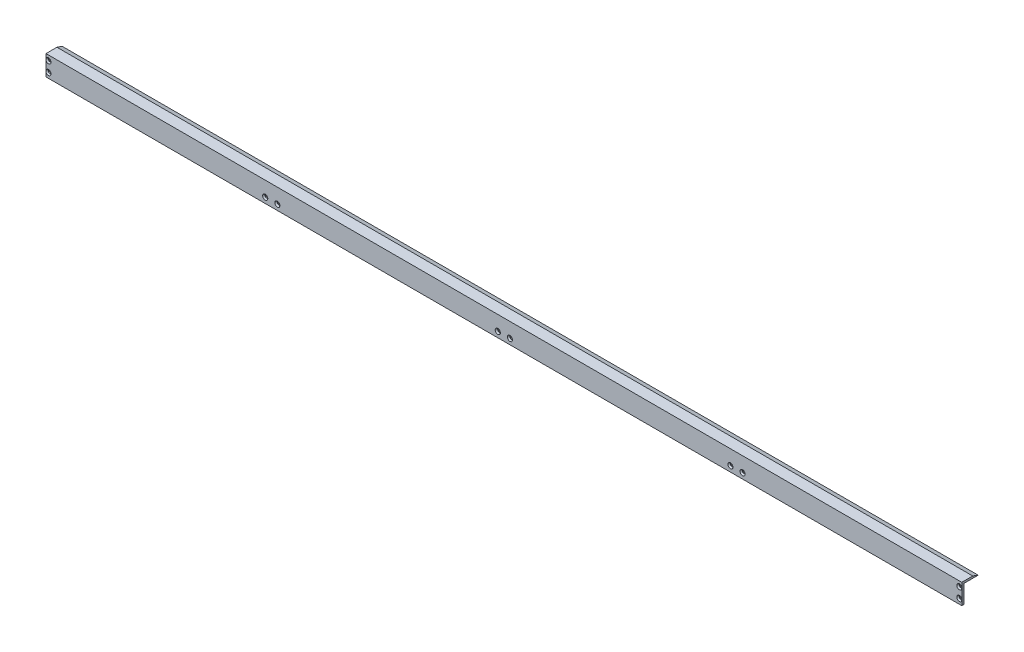
SolidWorks part; units mm, degrees
ref_plane "Front Plane" through (0, 0, 0) normal (0, 0, 1) x (1, 0, 0)
ref_plane "Top Plane" through (0, 0, 0) normal (0, 1, 0) x (1, 0, 0)
ref_plane "Right Plane" through (0, 0, 0) normal (1, 0, 0) x (0, 0, -1)
other "Configuration Table"
sketch "Sketch1" plane through (0, 0, 0) normal (0, 0, 1) x (1, 0, 0)
  line L1 (-1130, 25) -> (1130, 25)
  line L2 (-1130, 25) -> (-1130, -25)
  line L3 (-1130, -25) -> (1130, -25)
  line L4 (1130, 25) -> (1130, -25)
  line L5 (-1130, 25) -> (1130, -25) construction
  line L6 (-1130, -25) -> (1130, 25) construction
  point P0 (0, 0)
  dimension "D1" = 2260
  dimension "D2" = 50
extrude "Boss-Extrude1" add sketch "Sketch1" along normal blind 5
sketch "Sketch2" plane through (-1130, 0, 0) normal (-1, 0, 0) x (0, 0, 1)
  line L0 (5, 25) -> (5, -25) construction
  line L1 (0, 25) -> (-22, 25)
  line L2 (0, 25) -> (0, 20)
  line L3 (0, 20) -> (-35, 20)
  line L4 (-35, 20.5) -> (-35, 20)
  line L5 (-35, 20.5) -> (-22, 25)
  dimension "D1" = 5
  dimension "D2" = 40
  dimension "D3" = 0.5
  dimension "D4" = 13
extrude "Boss-Extrude2" add sketch "Sketch2" against normal up to vertex (2260 mm away) up to point (1130, 25, 0)
sketch "Sketch3" plane through (0, 0, 5) normal (0, 0, 1) x (1, 0, 0)
  line L0 (-1130, -25) -> (1130, -25) construction
  line L1 (-1130, 25) -> (-1130, -25) construction
  line L2 (1130, -25) -> (1130, 25) construction
  point P0 (-589, -11.3068)
  point P1 (-559, -11.3068)
  point P3 (-15, -11.3068)
  point P5 (15, -11.3068)
  point P7 (559, -11.3068)
  point P9 (589, -11.3068)
  point P14 (-1124, -12.5)
  point P16 (-1124, 12.5)
  point P23 (1124, -12.5)
  point P25 (1124, 12.5)
  dimension "D1" = 25
  dimension "D2" = 12.5
  dimension "D3" = 6
  dimension "D4" = 6
  dimension "D5" = 6
  dimension "D6" = 6
  dimension "D7" = 12.5
  dimension "D8" = 25
hole_wizard "CSK for M6 Hexagon lobular socket raised CTSK head screws1" positions "Sketch3" profile "Sketch4" countersink size "M6" standard "GB"
sketch "Sketch4" plane through (-589, -11.3068, 5) normal (1, 0, 0) x (0, -1, 0)
  line L0 (0, 0) -> (0, 21.7328)
  line L1 (0, 21.7328) -> (3.3, 19.75)
  line L2 (3.3, 19.75) -> (3.3, 3.1)
  line L3 (3.3, 3.1) -> (6.4, 0)
  line L5 (6.4, 0) -> (0, 0)
  line L6 (-3.3, 3.1) -> (-6.4, 0) construction
  line L10 (0, 21.7328) -> (-3.3, 19.75) construction
  line L11 (0, -6.35) -> (0, 107.95) construction
  dimension "孔直径" = 6.6
  dimension "孔深度" = 19.75
  dimension "近端锥形沉头孔直径" = 12.8
  dimension "近端锥形沉头孔角度" = 90
  dimension "导头角度" = 118
